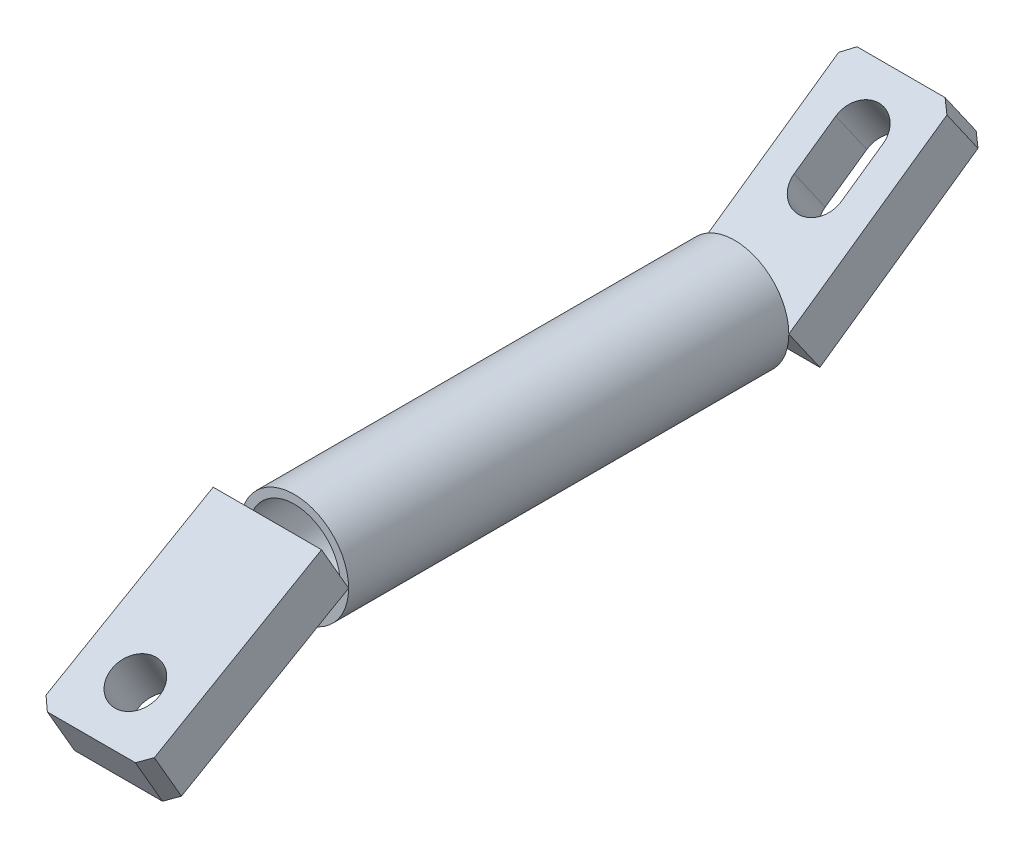
from build123d import *

# Parameters (mm, degrees)
SKETCH_1_R          = 16
SKETCH_1_R_2        = 13.5
EXTRUDE_1_DEPTH     = 130
EXTRUDE_2_DEPTH     = 16
CUT_EXTRUDE_1_DEPTH = 136.426599093
EXTRUDE_3_DEPTH     = 16
SKETCH_5_R          = 7
CUT_EXTRUDE_2_DEPTH = 181.267525325
CHAMFER_1_SIZE      = 3
CHAMFER_2_SIZE      = 3


with BuildPart() as part:
    # 草图1 → 凸台-拉伸1 (new body)
    with BuildSketch(Plane.XY):
        Circle(SKETCH_1_R)
        Circle(SKETCH_1_R_2, mode=Mode.SUBTRACT)
    extrude(amount=EXTRUDE_1_DEPTH)


with BuildPart() as body_2:
    # 草图2 → 凸台-拉伸2 (new, symmetric)
    with BuildSketch(Plane(origin=(0, 0, 0), x_dir=(0, 0, -1), z_dir=(1, 0, 0))):
        Polygon((0, 0), (49.149122657, 34.414586181), (58.326345639, 21.308153472), (9.177222982, -13.106432709), align=None)
    extrude(amount=EXTRUDE_2_DEPTH, both=True)

    # 草图3 → 切除-拉伸1 (cut, through all)
    with BuildSketch(Plane(origin=(0, 0, 0), x_dir=(1, 0, 0), z_dir=(0, 0.8191520442889908, 0.5735764363510477))):
        with BuildLine():
            Line((7, 45), (7, 30))
            ThreePointArc((7, 30), (0, 23), (-7, 30))
            Line((-7, 30), (-7, 45))
            ThreePointArc((-7, 45), (0, 52), (7, 45))
        make_face()
    extrude(amount=-CUT_EXTRUDE_1_DEPTH, mode=Mode.SUBTRACT)

    # 倒角2
    chamfer_2_edges = [body_2.edges().sort_by_distance(p)[0] for p in [
        (16, 27.861369827, -53.737734148),
        (-16, 27.861369827, -53.737734148),
    ]]
    chamfer(chamfer_2_edges, length=CHAMFER_2_SIZE)


with BuildPart() as body_3:
    # 草图4 → 凸台-拉伸3 (new, symmetric)
    with BuildSketch(Plane(origin=(0, 0, 0), x_dir=(0, 0, -1), z_dir=(1, 0, 0))):
        Polygon((-189.961524227, -16.143593539), (-181.961524227, -30), (-130, 0), (-138, 13.856406461), align=None)
    extrude(amount=EXTRUDE_3_DEPTH, both=True)

    # 草图5 → 切除-拉伸2 (cut, through all)
    with BuildSketch(Plane(origin=(0, 56.291651246, 32.5), x_dir=(1, 0, 0), z_dir=(0, -0.8660254037844374, -0.5000000000000021))):
        with Locations(Location((0, 157.583302492, 0), (0, 0, 270))):
            Circle(SKETCH_5_R)
    extrude(amount=-CUT_EXTRUDE_2_DEPTH, mode=Mode.SUBTRACT)

    # 倒角1
    chamfer_1_edges = [body_3.edges().sort_by_distance(p)[0] for p in [
        (16, -23.07179677, 185.961524227),
        (-16, -23.07179677, 185.961524227),
    ]]
    chamfer(chamfer_1_edges, length=CHAMFER_1_SIZE)


solid = Compound([part.part, body_2.part, body_3.part])
